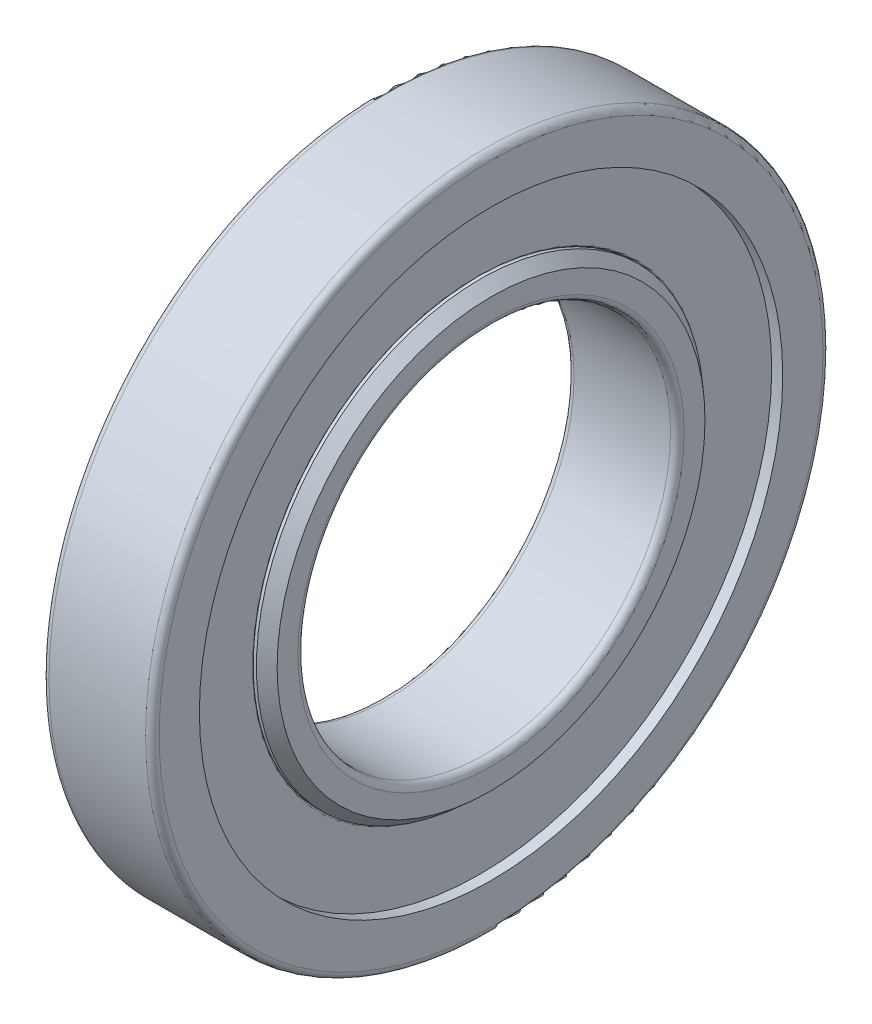
from build123d import *


with BuildPart() as part:
    # OutRacSke → OuterRace (revolve)
    with BuildSketch(Plane.XY, mode=Mode.PRIVATE) as outerrace_sk:
        with BuildLine():
            Line((-26, 172.2125), (-32.5, 172.2125))
            Line((-32.5, 172.2125), (-32.5, 196))
            ThreePointArc((-32.5, 196), (-31.328427125, 198.828427125), (-28.5, 200))
            Line((-28.5, 200), (28.5, 200))
            ThreePointArc((28.5, 200), (31.328427125, 198.828427125), (32.5, 196))
            Line((32.5, 196), (32.5, 172.2125))
            Line((32.5, 172.2125), (26, 172.2125))
            Line((26, 172.2125), (26, 177.95))
            Line((26, 177.95), (-26, 177.95))
            Line((-26, 177.95), (-26, 172.2125))
        make_face()
    revolve(outerrace_sk.sketch.rotate(Axis((-90, 0, 0), (1, 0, 0)), 270), axis=Axis((-90, 0, 0), (1, 0, 0)))

    # RolSimSke → RollersSimplified (revolve)
    with BuildSketch(Plane(origin=(0, 101.6, 0), x_dir=(1, 0, 0), z_dir=(0, 0, 1)), mode=Mode.PRIVATE) as rollerssimplified_sk:
        with BuildLine():
            Line((-24.7, 75.4368), (-24.7, 31.3632))
            ThreePointArc((-24.7, 31.3632), (-24.431065446, 30.713934554), (-23.7818, 30.445))
            Line((-23.7818, 30.445), (23.7818, 30.445))
            ThreePointArc((23.7818, 30.445), (24.431065446, 30.713934554), (24.7, 31.3632))
            Line((24.7, 31.3632), (24.7, 75.4368))
            ThreePointArc((24.7, 75.4368), (24.431065446, 76.086065446), (23.7818, 76.355))
            Line((23.7818, 76.355), (-23.7818, 76.355))
            ThreePointArc((-23.7818, 76.355), (-24.431065446, 76.086065446), (-24.7, 75.4368))
        make_face()
    revolve(rollerssimplified_sk.sketch.rotate(Axis((25.4, 0, 0), (-1, 0, 0)), 90), axis=Axis((25.4, 0, 0), (-1, 0, 0)))

    # InsRacSke → InnerRace (revolve)
    with BuildSketch(Plane.XY, mode=Mode.PRIVATE) as innerrace_sk:
        with BuildLine():
            Line((-26, 132.05), (-32.5, 126.3125))
            Line((-32.5, 126.3125), (-32.5, 114))
            ThreePointArc((-32.5, 114), (-31.328427125, 111.171572875), (-28.5, 110))
            Line((-28.5, 110), (28.5, 110))
            ThreePointArc((28.5, 110), (31.328427125, 111.171572875), (32.5, 114))
            Line((32.5, 114), (32.5, 126.3125))
            Line((32.5, 126.3125), (26, 132.05))
            Line((26, 132.05), (-26, 132.05))
        make_face()
    revolve(innerrace_sk.sketch.rotate(Axis((-90, 0, 0), (1, 0, 0)), 270), axis=Axis((-90, 0, 0), (1, 0, 0)))


solid = part.part
